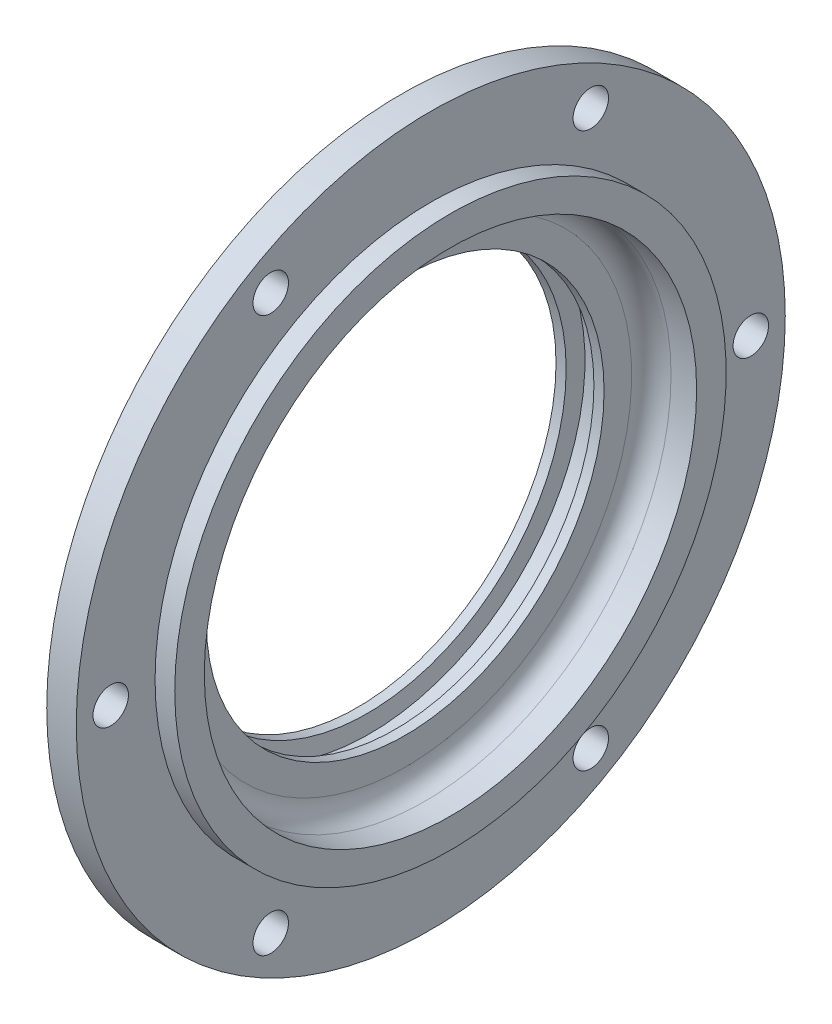
from build123d import *

# Parameters (mm, degrees)
SKETCH2_R          = 9
CUT_EXTRUDE1_DEPTH = 267.167044388


with BuildPart() as part:
    # Sketch1 → Revolve1 (revolve)
    with BuildSketch(Plane(origin=(0, 0, 0), x_dir=(1, 0, 0), z_dir=(0, 1, 0)), mode=Mode.PRIVATE) as revolve1_sk:
        with BuildLine():
            ThreePointArc((9235.135431533, 137.473726826), (9228.064363722, 134.544794638), (9225.135431533, 127.473726826))
            Line((9225.135431533, 127.473726826), (9225.135431533, 113.473726826))
            Line((9225.135431533, 113.473726826), (9219.979100301, 113.473726826))
            Line((9219.979100301, 113.473726826), (9218.935431533, 121.973726826))
            Line((9218.935431533, 121.973726826), (9206.935431533, 121.973726826))
            Line((9206.935431533, 121.973726826), (9205.891762766, 113.473726826))
            Line((9205.891762766, 113.473726826), (9200.735431533, 113.473726826))
            Line((9200.735431533, 113.473726826), (9200.735431533, 142.473726826))
            ThreePointArc((9200.735431533, 142.473726826), (9203.664363722, 149.544794638), (9210.735431533, 152.473726826))
            Line((9210.735431533, 152.473726826), (9213.135431533, 152.473726826))
            ThreePointArc((9213.135431533, 152.473726826), (9220.206499345, 155.402659014), (9223.135431533, 162.473726826))
            Line((9223.135431533, 162.473726826), (9223.135431533, 192.473726826))
            Line((9223.135431533, 192.473726826), (9238.135431533, 192.473726826))
            Line((9238.135431533, 192.473726826), (9238.135431533, 152.473726826))
            Line((9238.135431533, 152.473726826), (9248.135431533, 152.473726826))
            Line((9248.135431533, 152.473726826), (9248.135431533, 137.473726826))
            Line((9248.135431533, 137.473726826), (9235.135431533, 137.473726826))
        make_face()
    revolve(revolve1_sk.sketch.rotate(Axis((9092.86993426, 0, -12.473726826), (1, 0, 0)), 180), axis=Axis((9092.86993426, 0, -12.473726826), (1, 0, 0)))

    # Sketch2 → Cut-Extrude1 (cut, through all)
    with BuildSketch(Plane(origin=(9238.135431533, 0, 0), x_dir=(0, 0, -1), z_dir=(1, 0, 0))):
        with Locations((-68.776273174, 140.729128115)):
            Circle(SKETCH2_R)
        with Locations((93.723726826, 140.729128115)):
            Circle(SKETCH2_R)
        with Locations((174.973726826, 0)):
            Circle(SKETCH2_R)
        with Locations((93.723726826, -140.729128115)):
            Circle(SKETCH2_R)
        with Locations((-68.776273174, -140.729128115)):
            Circle(SKETCH2_R)
        with Locations((-150.026273174, 0)):
            Circle(SKETCH2_R)
    extrude(amount=-CUT_EXTRUDE1_DEPTH, mode=Mode.SUBTRACT)


solid = part.part
